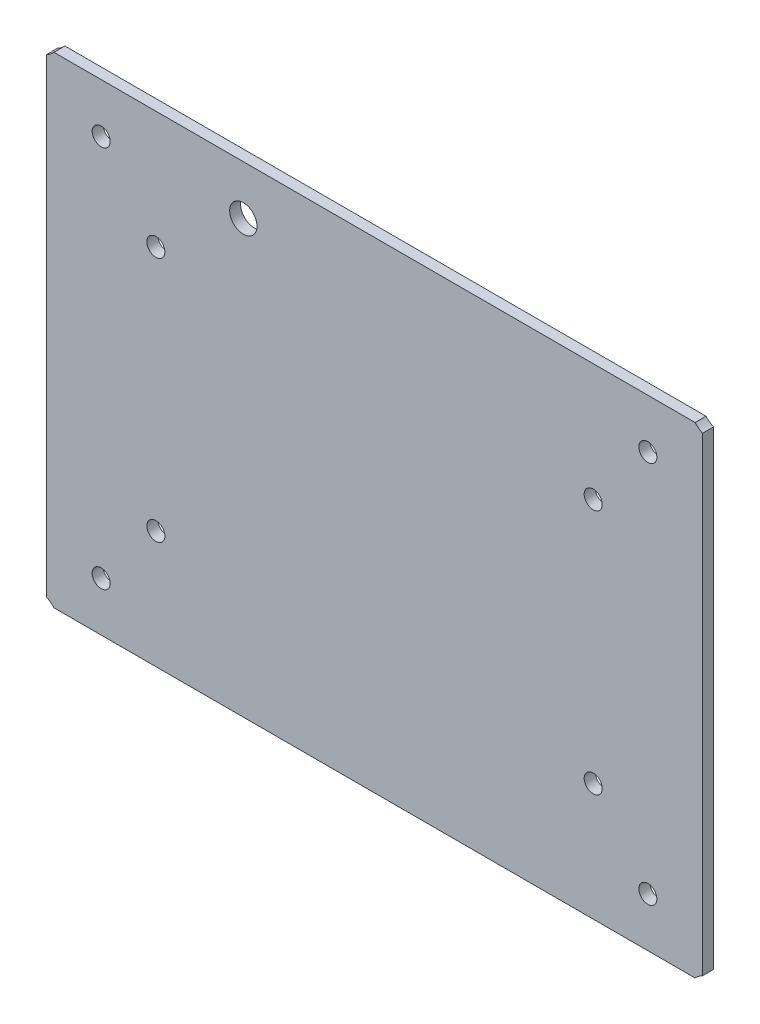
SolidWorks part; units mm, degrees
ref_plane "前视基准面" through (0, 0, 0) normal (0, 0, 1) x (1, 0, 0)
ref_plane "上视基准面" through (0, 0, 0) normal (0, 1, 0) x (1, 0, 0)
ref_plane "右视基准面" through (0, 0, 0) normal (1, 0, 0) x (0, 0, -1)
other "Configuration Table"
sketch "草图1" plane through (0, 0, 0) normal (0, 0, 1) x (1, 0, 0)
  line L0 (-60, -44) -> (60, -44)
  line L1 (60, -44) -> (60, 44)
  line L2 (60, 44) -> (-60, 44)
  line L3 (-60, 44) -> (-60, -44)
  circle A0 centre (-40, -22.5) radius 1.65
  circle A1 centre (-40, 22.5) radius 1.65
  circle A2 centre (40, -22.5) radius 1.65
  circle A3 centre (40, 22.5) radius 1.65
  circle A4 centre (-50, -35) radius 1.65
  circle A5 centre (-50, 35) radius 1.65
  circle A6 centre (50, -35) radius 1.65
  circle A7 centre (50, 35) radius 1.65
  circle A8 centre (-24, 35) radius 2.5
  point P0 (0, 0)
  dimension "D1" = 3.3
  dimension "D2" = 3.3
  dimension "D3" = 3.3
  dimension "D4" = 3.3
  dimension "D5" = 3.3
  dimension "D6" = 5
  dimension "D7" = 3.3
  dimension "D8" = 3.3
  dimension "D9" = 3.3
  dimension "D10" = 10
  dimension "D11" = 20
  dimension "D12" = 60
  dimension "D13" = 84
  dimension "D14" = 100
  dimension "D15" = 110
  dimension "D16" = 120
  dimension "D17" = 9
  dimension "D18" = 21.5
  dimension "D19" = 44
  dimension "D20" = 66.5
  dimension "D21" = 79
  dimension "D22" = 88
extrude "凸台-拉伸1" add sketch "草图1" against normal mid plane 2
sketch "草图2" plane through (0, 0, 0) normal (0, 0, 1) x (1, 0, 0)
  circle A0 centre (-62, -47) radius 4.5
  circle A1 centre (-62, 47) radius 4.5
  circle A2 centre (62, -47) radius 4.5
  circle A3 centre (62, 47) radius 4.5
  point P0 (0, 0)
  dimension "D1" = 9
  dimension "D2" = 9
  dimension "D3" = 9
  dimension "D4" = 9
  dimension "D5" = 62
  dimension "D6" = 124
  dimension "D7" = 47
  dimension "D8" = 94
extrude "切除-拉伸1" cut sketch "草图2" against normal mid plane 5
